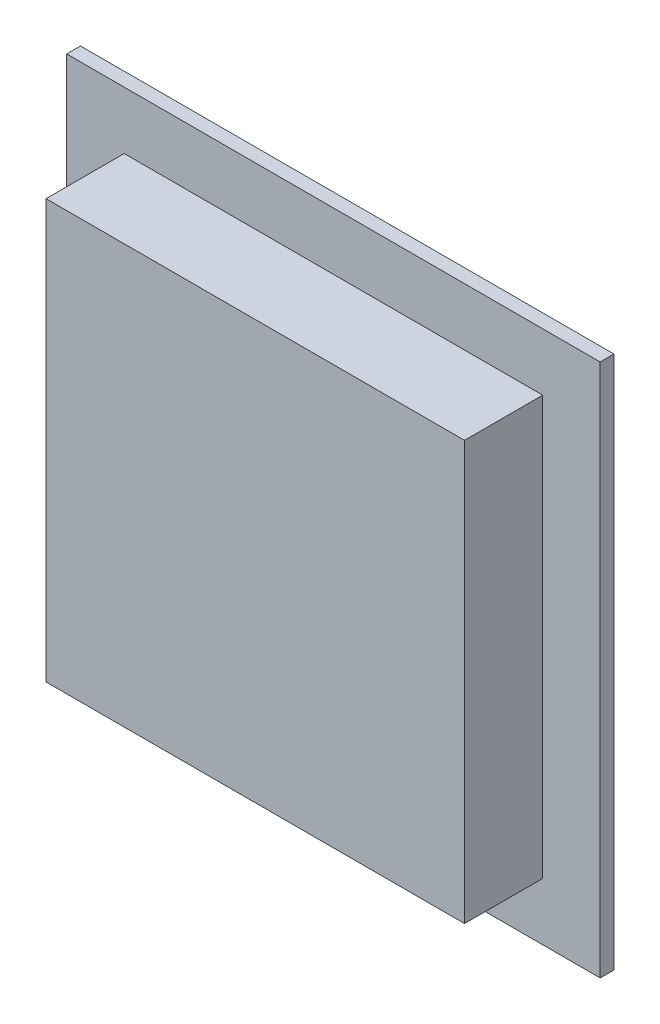
SolidWorks part; units mm, degrees
ref_plane "前视基准面" through (0, 0, 0) normal (0, 0, 1) x (1, 0, 0)
ref_plane "上视基准面" through (0, 0, 0) normal (0, 1, 0) x (1, 0, 0)
ref_plane "右视基准面" through (0, 0, 0) normal (1, 0, 0) x (0, 0, -1)
sketch "草图1" plane through (0, 0, 0) normal (0, 0, 1) x (1, 0, 0)
  line L1 (-58, 58) -> (58, 58)
  line L2 (-58, 58) -> (-58, -58)
  line L3 (-58, -58) -> (58, -58)
  line L4 (58, 58) -> (58, -58)
  line L5 (-58, 58) -> (58, -58) construction
  line L6 (-58, -58) -> (58, 58) construction
  point P0 (0, 0)
  dimension "D1" = 116
  dimension "D2" = 116
extrude "凸台-拉伸1" add sketch "草图1" along normal blind 3
sketch "草图2" plane through (0, 0, 3) normal (0, 0, 1) x (1, 0, 0)
  line L1 (-45.5, 45.5) -> (45.5, 45.5)
  line L2 (-45.5, 45.5) -> (-45.5, -45.5)
  line L3 (-45.5, -45.5) -> (45.5, -45.5)
  line L4 (45.5, 45.5) -> (45.5, -45.5)
  line L5 (-45.5, 45.5) -> (45.5, -45.5) construction
  line L6 (-45.5, -45.5) -> (45.5, 45.5) construction
  point P0 (0, 0)
  dimension "D1" = 91
extrude "凸台-拉伸2" add sketch "草图2" along normal blind 17
